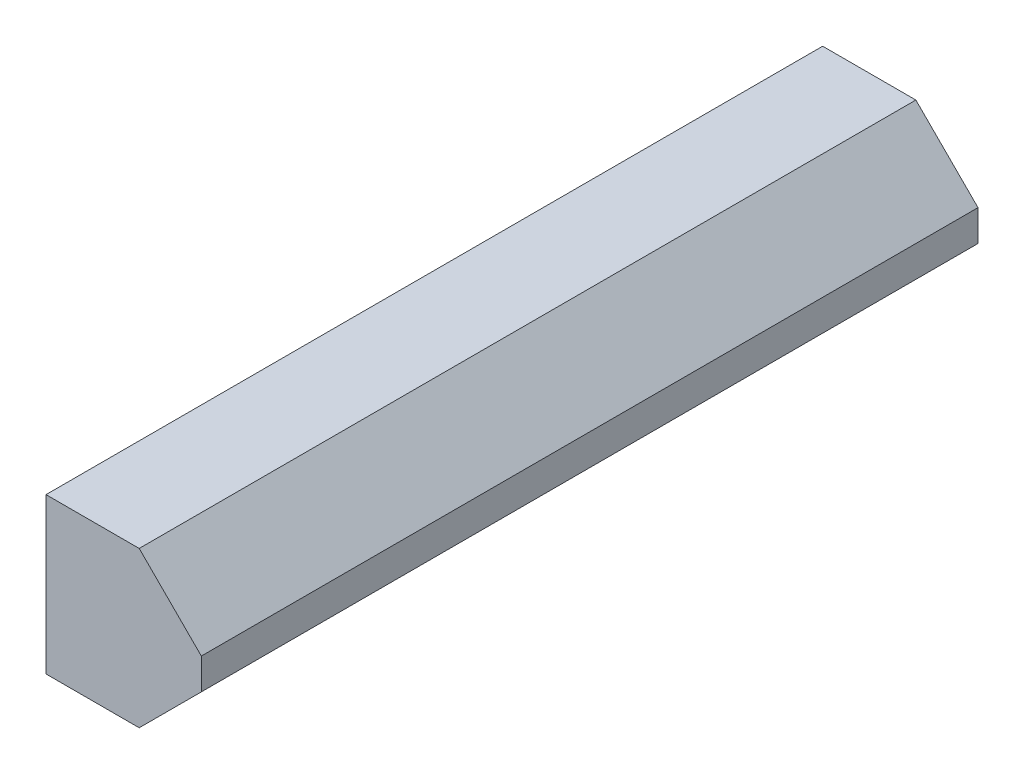
SolidWorks part; units mm, degrees
material "Q235-A"
ref_plane "Front Plane" through (0, 0, 0) normal (0, 0, 1) x (1, 0, 0)
ref_plane "Top Plane" through (0, 0, 0) normal (0, 1, 0) x (1, 0, 0)
ref_plane "Right Plane" through (0, 0, 0) normal (1, 0, 0) x (0, 0, -1)
sketch "Sketch1" plane through (0, 0, 0) normal (1, 0, 0) x (0, 0, -1)
  line L1 (125, -25) -> (-125, -25)
  line L2 (125, -25) -> (125, 25)
  line L3 (125, 25) -> (-125, 25)
  line L4 (-125, -25) -> (-125, 25)
  line L5 (125, -25) -> (-125, 25) construction
  line L6 (125, 25) -> (-125, -25) construction
  point P0 (0, 0)
  dimension "D1" = 50
  dimension "D2" = 250
extrude "Boss-Extrude1" add sketch "Sketch1" along normal mid plane 50
chamfer "Chamfer1" distance 20 angle 45 2 edges at (25, -25, 0) (25, 25, 0)
